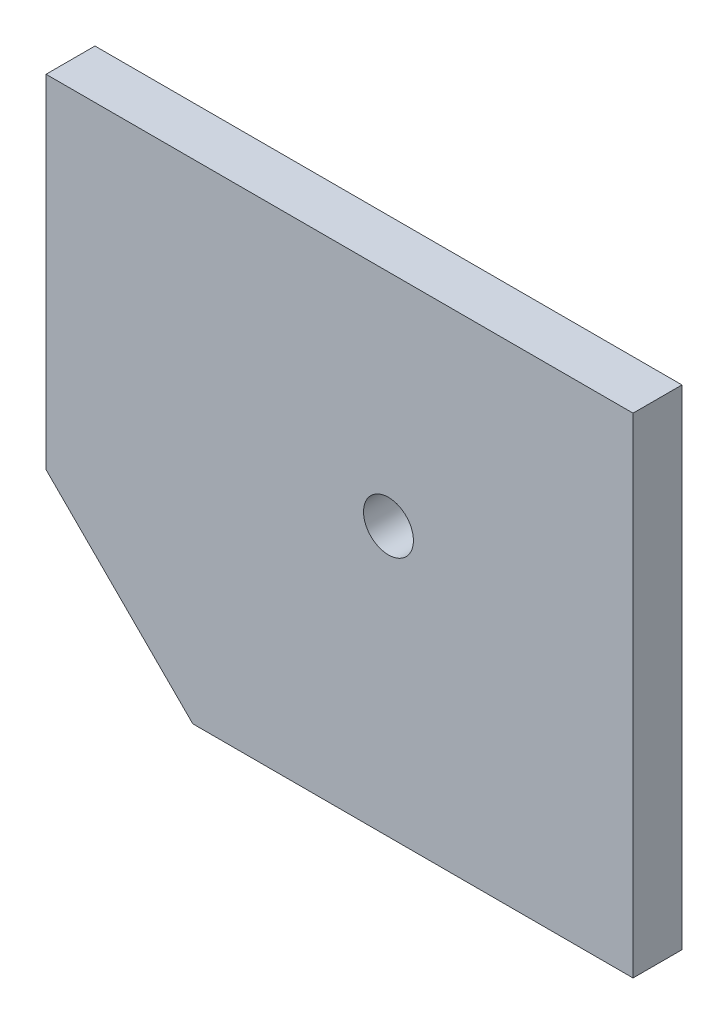
from build123d import *

# Parameters (mm, degrees)
EXTRUDE_1_DEPTH         = 10
HOLE_WIZARD_M12_1_D     = 10.2
HOLE_WIZARD_M12_1_DEPTH = 32.75
HOLE_WIZARD_M12_1_TIP   = 3.064389157


with BuildPart() as part:
    # 草图1 → 凸台-拉伸1 (new body)
    with BuildSketch(Plane.XY):
        Polygon((-30.845070423, -49.295774648), (-60.845070423, -19.295774648), (-60.845070423, 50.704225352), (59.154929577, 50.704225352), (59.154929577, -49.295774648), align=None)
    extrude(amount=EXTRUDE_1_DEPTH)

    # M12 螺纹孔1
    with Locations(Plane.XY.offset(10)):
        with Locations((9.154929577, 5.704225352)):
            Hole(HOLE_WIZARD_M12_1_D / 2, depth=HOLE_WIZARD_M12_1_DEPTH)
            with Locations((0, 0, -(HOLE_WIZARD_M12_1_DEPTH + HOLE_WIZARD_M12_1_TIP / 2))):  # 118° drill point
                Cone(0, HOLE_WIZARD_M12_1_D / 2, HOLE_WIZARD_M12_1_TIP, mode=Mode.SUBTRACT)


solid = part.part
